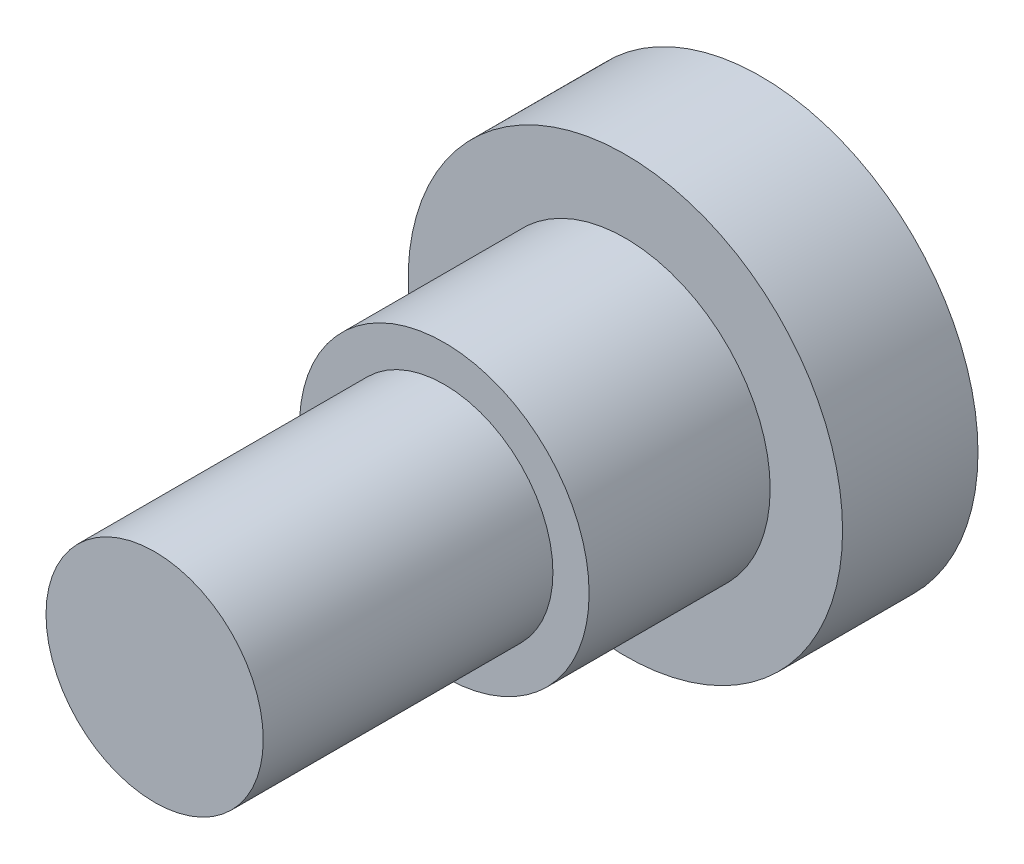
from build123d import *

# Parameters (mm, degrees)
SKETCH_1_R      = 6
EXTRUDE_1_DEPTH = 3.74
SKETCH_2_R      = 4
EXTRUDE_2_DEPTH = 5
SKETCH_3_R      = 3
EXTRUDE_3_DEPTH = 8


with BuildPart() as part:
    # 草图1 → 凸台-拉伸1 (new body)
    with BuildSketch(Plane.XY):
        Circle(SKETCH_1_R)
    extrude(amount=EXTRUDE_1_DEPTH)

    # 草图2 → 凸台-拉伸2 (add)
    with BuildSketch(Plane.XY.offset(3.74)):
        Circle(SKETCH_2_R)
    extrude(amount=EXTRUDE_2_DEPTH)

    # 草图3 → 凸台-拉伸3 (add)
    with BuildSketch(Plane.XY.offset(8.74)):
        Circle(SKETCH_3_R)
    extrude(amount=EXTRUDE_3_DEPTH)


solid = part.part
